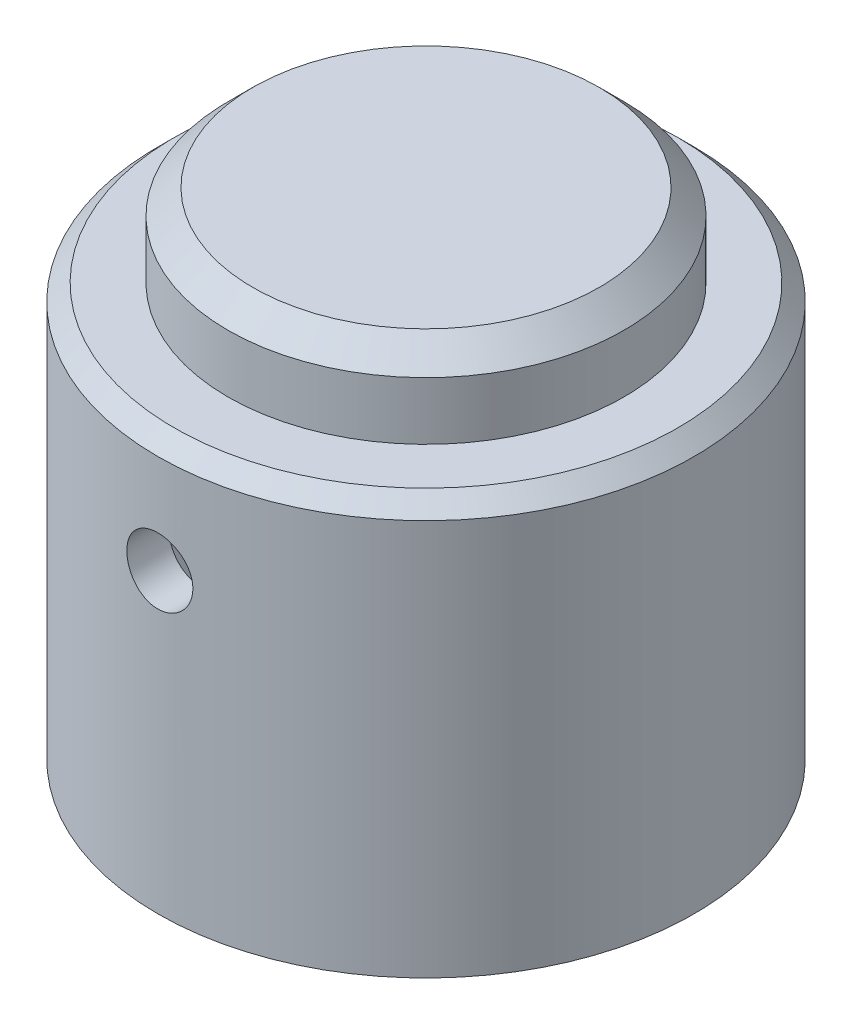
SolidWorks part; units mm, degrees
ref_plane "Front Plane" through (0, 0, 0) normal (0, 0, 1) x (1, 0, 0)
ref_plane "Top Plane" through (0, 0, 0) normal (0, 1, 0) x (1, 0, 0)
ref_plane "Right Plane" through (0, 0, 0) normal (1, 0, 0) x (0, 0, -1)
sketch "Sketch1" plane through (0, 0, 0) normal (0, 0, 1) x (1, 0, 0)
  line L0 (0, 0) -> (0, 60) construction
  line L1 (0, 60) -> (-24, 60)
  line L2 (-24, 60) -> (-24, 50)
  line L3 (-24, 50) -> (-32.5, 50)
  line L4 (-32.5, 50) -> (-32.5, 0)
  line L5 (-32.5, 0) -> (0, 0)
  line L6 (0, 0) -> (0, 60)
  dimension "D1" = 32.5
  dimension "D2" = 24
  dimension "D3" = 10
  dimension "D4" = 60
revolve "Revolve1" add sketch "Sketch1" angle 360 about L0
chamfer "Chamfer1" distance 3 angle 45 1 edges at (0, 60, -24)
chamfer "Chamfer2" distance 2 angle 45 1 edges at (0, 50, -32.5)
sketch "Sketch2" plane through (0, 0, 0) normal (0, 0, 1) x (1, 0, 0)
  line L0 (-27.5, 0) -> (-27.5, 40)
  line L1 (-32.5, 0) -> (32.5, 0) construction
  line L2 (-27.5, 40) -> (-15, 40)
  line L3 (-15, 40) -> (-15, 38)
  line L4 (-15, 38) -> (0, 38)
  line L5 (0, 0) -> (-27.5, 0)
  line L6 (30.5, 50) -> (-30.5, 50) construction
  line L7 (0, 38) -> (0, 0)
  line L8 (0, 38) -> (0, 0) construction
  dimension "D1" = 12
  dimension "D2" = 27.5
  dimension "D3" = 2
  dimension "15" = 15
revolve "Cut-Revolve1" cut sketch "Sketch2" angle 360 about L8
sketch "Sketch3" plane through (0, 0, 0) normal (0, 0, 1) x (1, 0, 0)
  circle A0 centre (0, 36) radius 4
  dimension "D2" = 8
  dimension "D1" = 36
extrude "Cut-Extrude1" cut sketch "Sketch3" against normal blind 105 from offset 20 offset against normal yes
sketch "Sketch4" plane through (0, 0, 0) normal (0, 0, 1) x (1, 0, 0)
  circle A0 centre (0, 36) radius 4
  dimension "D1" = 8
extrude "Cut-Extrude2" cut sketch "Sketch4" along normal blind 105 from offset 20
sketch "Sketch7" plane through (0, 0, 0) normal (1, 0, 0) x (0, 0, -1)
  line L0 (-5.375, 38) -> (-5.375, 50)
  line L1 (-15, 38) -> (15, 38) construction
  line L2 (-5.375, 50) -> (0, 53.1033)
  line L3 (0, 53.1033) -> (0, 0) construction
  line L4 (-5.375, 38) -> (0, 38)
  line L5 (0, 38) -> (0, 53.1033)
  dimension "D1" = 12
  dimension "D2" = 60
  dimension "D3" = 5.375
revolve "Cut-Revolve2" cut sketch "Sketch7" angle 360 about L3
